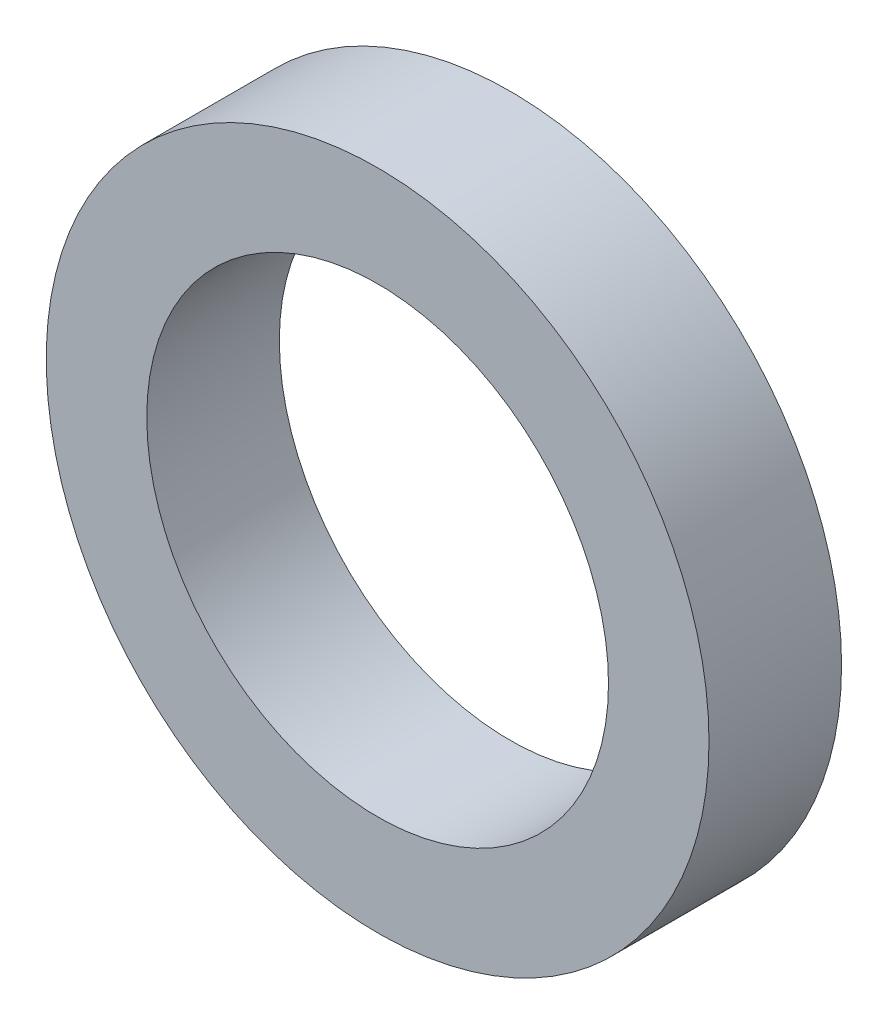
from build123d import *

# Parameters (mm, degrees)
SKETCH1_R           = 30
SKETCH1_R_2         = 20.9
BOSS_EXTRUDE1_DEPTH = 12


with BuildPart() as part:
    # Sketch1 → Boss-Extrude1 (new body)
    with BuildSketch(Plane.XY):
        Circle(SKETCH1_R)
        Circle(SKETCH1_R_2, mode=Mode.SUBTRACT)
    extrude(amount=BOSS_EXTRUDE1_DEPTH)


solid = part.part
